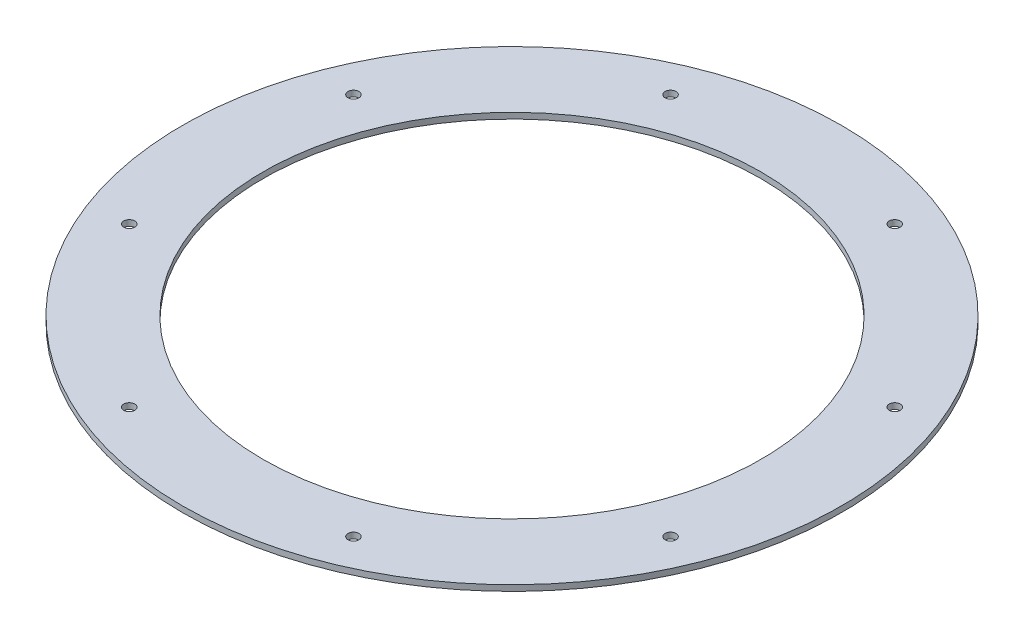
from build123d import *

# Parameters (mm, degrees)
SKETCH1_R                  = 450
SKETCH1_R_2                = 340
BOSS_EXTRUDE1_DEPTH        = 4
F_15_0_15_DIAMETER_HOLE1_D = 15


with BuildPart() as part:
    # Sketch1 → Boss-Extrude1 (new, symmetric)
    with BuildSketch(Plane(origin=(0, 0, 0), x_dir=(1, 0, 0), z_dir=(0, 1, 0))):
        with Locations(Location((0, 0, 0), (0, 0, 270))):
            Circle(SKETCH1_R)
        with Locations(Location((0, 0, 0), (0, 0, 270))):
            Circle(SKETCH1_R_2, mode=Mode.SUBTRACT)
    extrude(amount=BOSS_EXTRUDE1_DEPTH, both=True)

    # Ø15.0 (15) Diameter Hole1 (through all)
    with Locations(Plane(origin=(0, 4, 0), x_dir=(1, 0, 0), z_dir=(0, 1, 0))):
        with Locations((153.073372946, 369.551813005), (369.551813005, 153.073372946), (369.551813005, -153.073372946), (153.073372946, -369.551813005), (-153.073372946, -369.551813005), (-369.551813005, -153.073372946), (-369.551813005, 153.073372946), (-153.073372946, 369.551813005)):
            Hole(F_15_0_15_DIAMETER_HOLE1_D / 2)


solid = part.part
